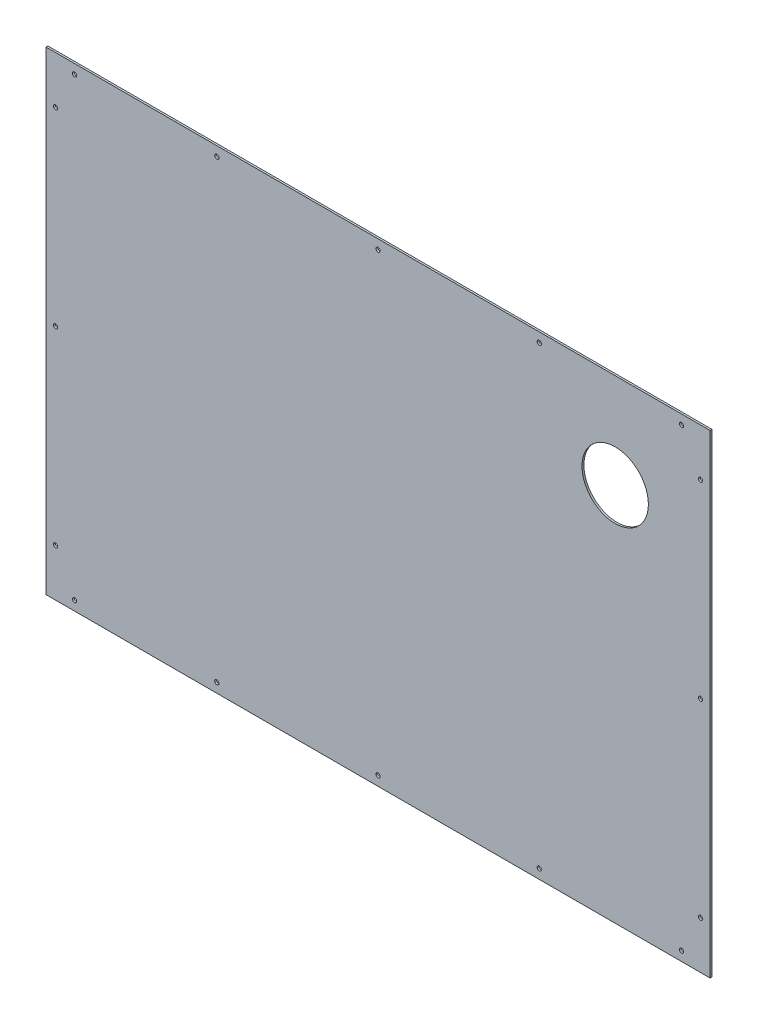
SolidWorks part; units mm, degrees
material "Q235A"
ref_plane "前视基准面" through (0, 0, 0) normal (0, 0, 1) x (1, 0, 0)
ref_plane "上视基准面" through (0, 0, 0) normal (0, 1, 0) x (1, 0, 0)
ref_plane "右视基准面" through (0, 0, 0) normal (1, 0, 0) x (0, 0, -1)
sketch "草图1" plane through (0, 0, 0) normal (0, 0, 1) x (1, 0, 0)
  line L1 (-350, 250) -> (350, 250)
  line L2 (-350, 250) -> (-350, -250)
  line L3 (-350, -250) -> (350, -250)
  line L4 (350, 250) -> (350, -250)
  line L5 (0, -250) -> (0, 250) construction
  line L6 (-350, 0) -> (350, 0) construction
  point P0 (0, 0)
  dimension "D1" = 700
  dimension "D2" = 500
extrude "凸台-拉伸1" add sketch "草图1" along normal blind 2
hole_wizard "Ø4.5 (4.5) 直径孔1" positions "草图2" profile "草图3" hole size "Ø4.5" standard "GB" end condition through all
sketch "草图2" plane through (0, 0, 2) normal (0, 0, 1) x (1, 0, 0)
  line L1 (-340, -240) -> (340, -240) construction
  line L2 (-340, -240) -> (-340, 240) construction
  line L3 (-340, 240) -> (340, 240) construction
  line L4 (340, -240) -> (340, 240) construction
  line L5 (0, 240) -> (0, -240) construction
  line L6 (-340, 0) -> (340, 0) construction
  line L7 (-320, 240) -> (-320, -240) construction
  line L9 (320, 240) -> (320, -240) construction
  point P305 (-340, 0)
  point P306 (0, -240)
  point P307 (340, 0)
  point P308 (0, 240)
  point P312 (-170, 240)
  point P324 (170, 240)
  point P329 (-170, -240)
  point P331 (170, -240)
  point P340 (-320, 240)
  point P342 (320, 240)
  point P345 (-340, 200)
  point P347 (-340, -200)
  point P349 (340, -200)
  point P351 (340, 200)
  point P354 (-320, -240)
  point P357 (320, -240)
  dimension "D1" = 680
  dimension "D2" = 480
  dimension "D3" = 170
  dimension "170" = 170
  dimension "D4" = 170
  dimension "D5" = 340
  dimension "D6" = 150
  dimension "D7" = 150
  dimension "D8" = 400
  dimension "D9" = 400
sketch "草图3" plane through (320, -240, 2) normal (1, 0, 0) x (0, -1, 0)
  line L0 (0, 0) -> (0, 2)
  line L1 (0, 2) -> (2.25, 2)
  line L2 (2.25, 2) -> (2.25, 0)
  line L5 (2.25, 0) -> (0, 0)
  line L11 (0, -6.35) -> (0, 107.95) construction
  dimension "通孔孔直径" = 4.5
  dimension "通孔孔深度" = 2
sketch "草图4" plane through (0, 0, 2) normal (0, 0, 1) x (1, 0, 0)
  line L0 (0, 250) -> (0, -250) construction
  line L1 (350, 250) -> (-350, 250) construction
  line L2 (-350, -250) -> (350, -250) construction
  line L3 (-350, 0) -> (353.8196, 0) construction
  line L4 (-350, 250) -> (-350, -250) construction
  line L5 (350, -250) -> (350, 250) construction
  circle A0 centre (250, 150) radius 35
  point P15 (250, 170.6096)
  dimension "D1" = 70
  dimension "D3" = 100
  dimension "D2" = 150
extrude "切除-拉伸1" cut sketch "草图4" against normal blind 10
